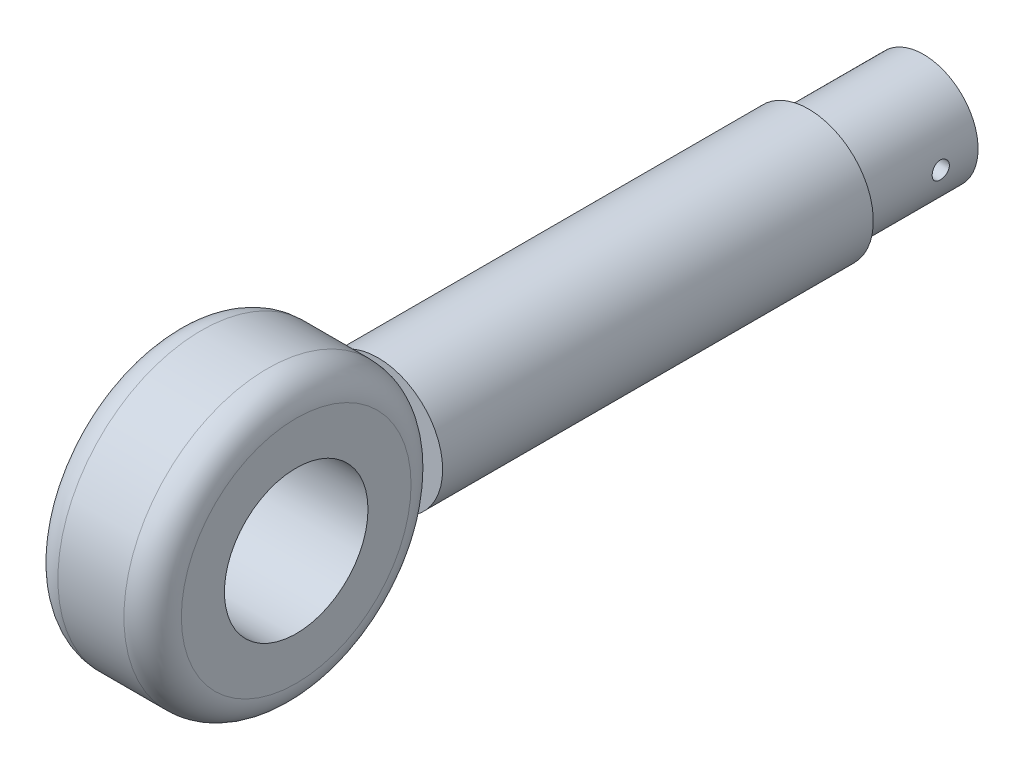
SolidWorks part; units mm, degrees
material "AISI 1045 钢，冷拔"
ref_plane "前视基准面" through (0, 0, 0) normal (0, 0, 1) x (1, 0, 0)
ref_plane "上视基准面" through (0, 0, 0) normal (0, 1, 0) x (1, 0, 0)
ref_plane "右视基准面" through (0, 0, 0) normal (1, 0, 0) x (0, 0, -1)
sketch "草图1" plane through (0, 0, 0) normal (0, 0, 1) x (1, 0, 0)
  circle A0 centre (0, 0) radius 22.5
  dimension "D1" = 45
extrude "凸台-拉伸1" add sketch "草图1" along normal blind 190
sketch "草图2" plane through (0, 0, 0) normal (1, 0, 0) x (0, 0, -1)
  line L0 (-190, 22.5) -> (-190, -22.5) construction
  circle A0 centre (-240, 0) radius 50
  circle A1 centre (-240, 0) radius 25
  dimension "D1" = 100
  dimension "D2" = 50
extrude "凸台-拉伸2" add sketch "草图2" along normal mid plane 43 separate body
fillet "圆角1" radius 10 2 edges at (-21.5, 0, 190) (21.5, 0, 190)
sketch "草图3" plane through (0, 0, 0) normal (0, 0, -1) x (-1, 0, 0)
  circle A0 centre (0, 0) radius 22.5
  circle A1 centre (0, 0) radius 19
  dimension "D1" = 45
  dimension "D2" = 38
extrude "切除-拉伸1" cut sketch "草图3" against normal blind 40
cosmetic thread "装饰螺纹线1"
sketch "草图4" plane through (0, 0, 0) normal (1, 0, 0) x (0, 0, -1)
  circle A0 centre (-13, 0) radius 3
  dimension "D2" = 6
  dimension "D1" = 13
extrude "切除-拉伸2" cut sketch "草图4" against normal mid plane 50
